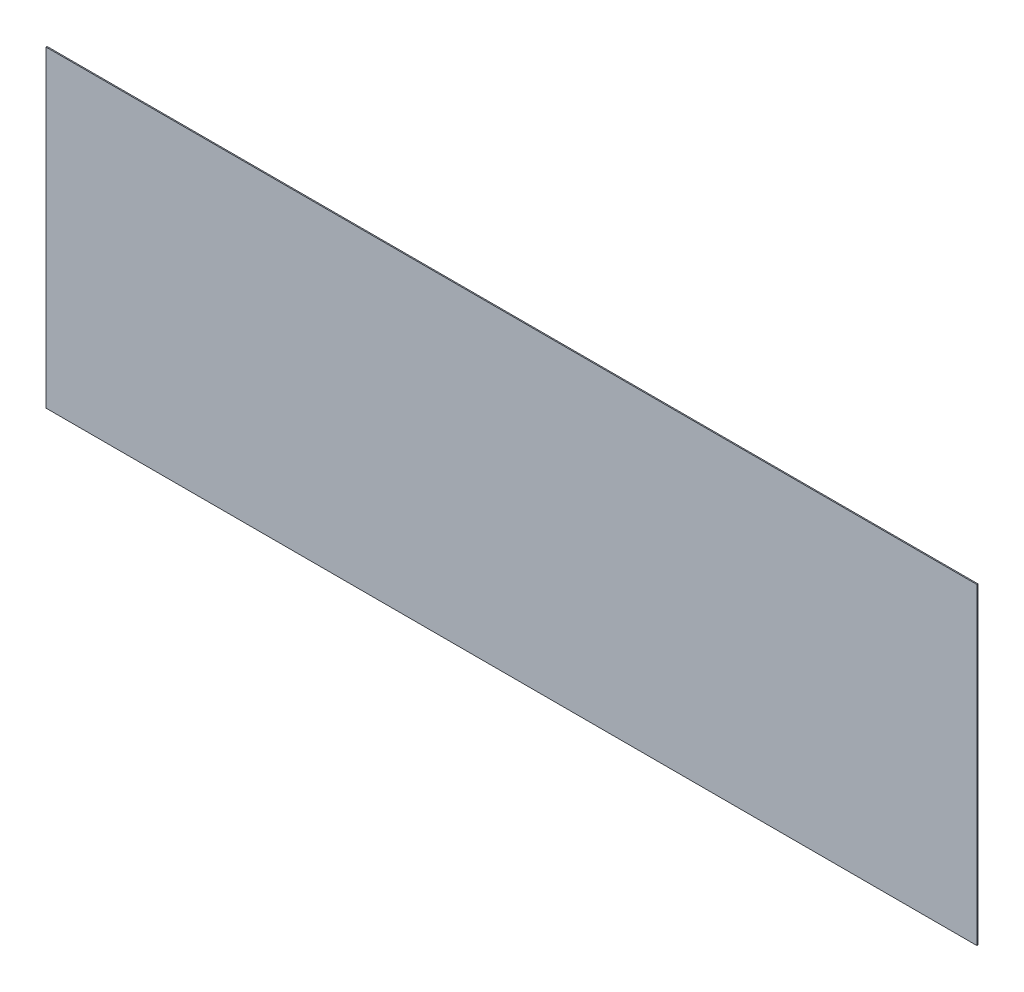
SolidWorks part; units mm, degrees
ref_plane "Front Plane" through (0, 0, 0) normal (0, 0, 1) x (1, 0, 0)
ref_plane "Top Plane" through (0, 0, 0) normal (0, 1, 0) x (1, 0, 0)
ref_plane "Right Plane" through (0, 0, 0) normal (1, 0, 0) x (0, 0, -1)
sketch "Sketch1" plane through (0, 0, 0) normal (0, 0, 1) x (1, 0, 0)
  line L1 (0, 0) -> (1280, 0)
  line L2 (0, 0) -> (0, 430)
  line L3 (0, 430) -> (1280, 430)
  line L4 (1280, 0) -> (1280, 430)
extrude "Boss-Extrude1" add sketch "Sketch1" along normal blind 1.5
